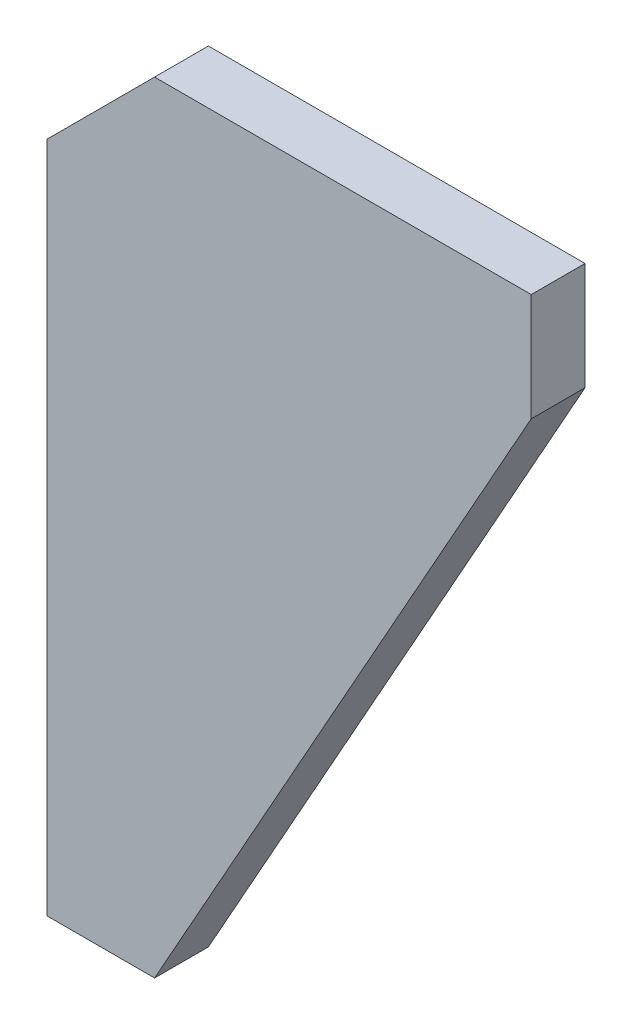
from build123d import *

# Parameters (mm, degrees)
BOSS_EXTRUDE1_DEPTH = 10


with BuildPart() as part:
    # Sketch1 → Boss-Extrude1 (new body)
    with BuildSketch(Plane.XY):
        Polygon((0, 0), (20, 0), (90, 125), (90, 145), (20, 145), (0, 125), align=None)
    extrude(amount=BOSS_EXTRUDE1_DEPTH)


solid = part.part
